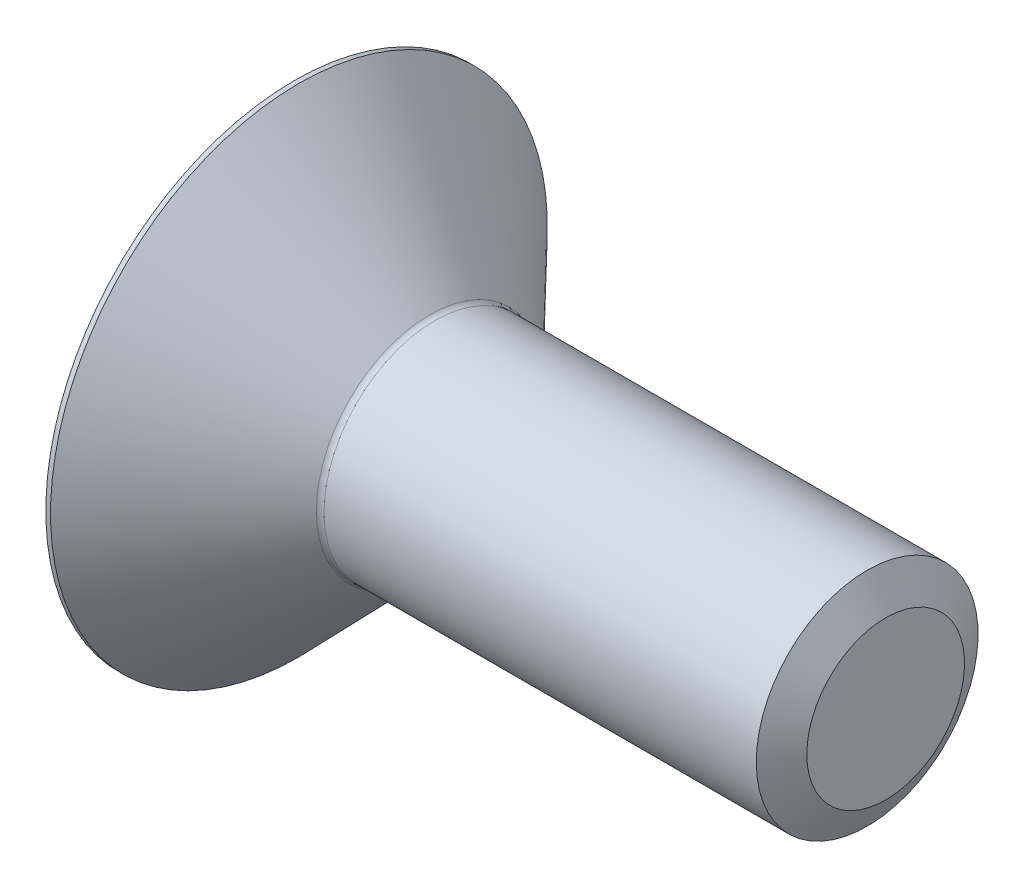
from build123d import *

# Parameters (mm, degrees)
CUT_EXTRUDE1_DEPTH = 1.96


with BuildPart() as part:
    # Sketch1 → Revolve1 (revolve)
    with BuildSketch(Plane.XY):
        with BuildLine():
            Line((0, 1.5), (-6.097552518, 1.5))
            ThreePointArc((-6.097552518, 1.5), (-6.136625631, 1.507949515), (-6.169486498, 1.530534163))
            Line((-6.169486498, 1.530534163), (-7.936181121, 3.36))
            Line((-7.936181121, 3.36), (-8, 3.36))
            Line((-8, 3.36), (-8, 0))
            Line((-8, 0), (0, 0))
            Line((0, 0), (0, 1.5))
        make_face()
    revolve(axis=Axis((0, 0, 0), (-1, 0, 0)))

    # Sketch2 → Cut-Extrude1 (cut)
    with BuildSketch(Plane.ZY.offset(8)):
        Polygon((0, 1.154700538), (-1, 0.577350269), (-1, -0.577350269), (0, -1.154700538), (1, -0.577350269), (1, 0.577350269), align=None)
    extrude(amount=-CUT_EXTRUDE1_DEPTH, mode=Mode.SUBTRACT)

    # Sketch6 → Revolve2 (revolve)
    with BuildSketch(Plane.XY, mode=Mode.PRIVATE) as revolve2_sk:
        Polygon((-6.9, 1.154700538), (-6.233333333, 0), (-5.74, 0), (-5.74, 1.154700538), align=None)
    revolve(revolve2_sk.sketch.rotate(Axis((-8, 0, 0), (1, 0, 0)), 90), axis=Axis((-8, 0, 0), (1, 0, 0)))

    # Sketch7 → Cut-Revolve2 (revolve, cut)
    with BuildSketch(Plane.XY):
        Polygon((-8, 1.154700538), (-8, 0), (-7.67, 0), align=None)
    revolve(axis=Axis((-8, 0, 0), (1, 0, 0)), mode=Mode.SUBTRACT)

    # Sketch4 → Cut-Revolve1 (revolve, cut)
    with BuildSketch(Plane.XY):
        Polygon((-0.25, 1.5), (0, 1.066987298), (0.25, 1.5), align=None)
    revolve(axis=Axis((-0.25, 0, 0), (1, 0, 0)), mode=Mode.SUBTRACT)


solid = part.part
